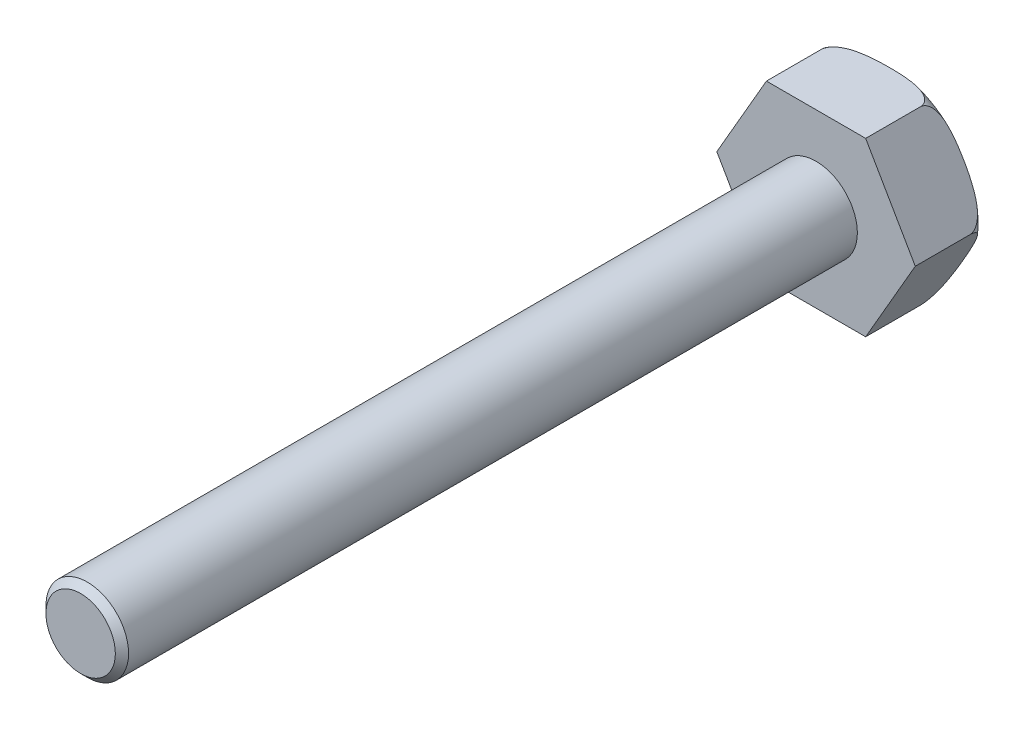
SolidWorks part; units mm, degrees
ref_plane "Front Plane" through (0, 0, 0) normal (0, 0, 1) x (1, 0, 0)
ref_plane "Top Plane" through (0, 0, 0) normal (0, 1, 0) x (1, 0, 0)
ref_plane "Right Plane" through (0, 0, 0) normal (1, 0, 0) x (0, 0, -1)
sketch "Sketch1" plane through (0, 0, 0) normal (0, 0, 1) x (1, 0, 0)
  line L1 (30.0222, -52) -> (60.0444, 0)
  line L2 (60.0444, 0) -> (30.0222, 52)
  line L3 (30.0222, 52) -> (-30.0222, 52)
  line L4 (-30.0222, 52) -> (-60.0444, 0)
  line L5 (-60.0444, 0) -> (-30.0222, -52)
  line L6 (-30.0222, -52) -> (30.0222, -52)
  circle A0 centre (0, 0) radius 52 construction
  dimension "D1" = 104
extrude "Boss-Extrude1" add sketch "Sketch1" along normal blind 45
sketch "Sketch3" plane through (0, 0, 0) normal (0, 1, 0) x (1, 0, 0)
  line L0 (0, 19.888) -> (0, -58.7862) construction
  line L1 (-60.0444, -45) -> (-60.0444, 0) construction
  line L2 (-30.0222, 0) -> (-60.0444, 0) construction
  line L3 (-60.0444, -12) -> (-60.0444, 0)
  line L4 (-60.0444, 0) -> (-48.0444, 0)
  arc A0 (-60.0444, -12) -> (-48.0444, 0) centre (-48.0444, -12) cw
  dimension "D1" = 12
revolve "Cut-Revolve3" cut sketch "Sketch3" angle 360 about L0
sketch "Sketch4" plane through (0, 0, 45) normal (0, 0, 1) x (1, 0, 0)
  circle A0 centre (0, 0) radius 25
  dimension "D1" = 50
extrude "Boss-Extrude2" add sketch "Sketch4" along normal blind 445
chamfer "Chamfer2" distance 4 angle 45 1 edges at (25, 0, 490)
